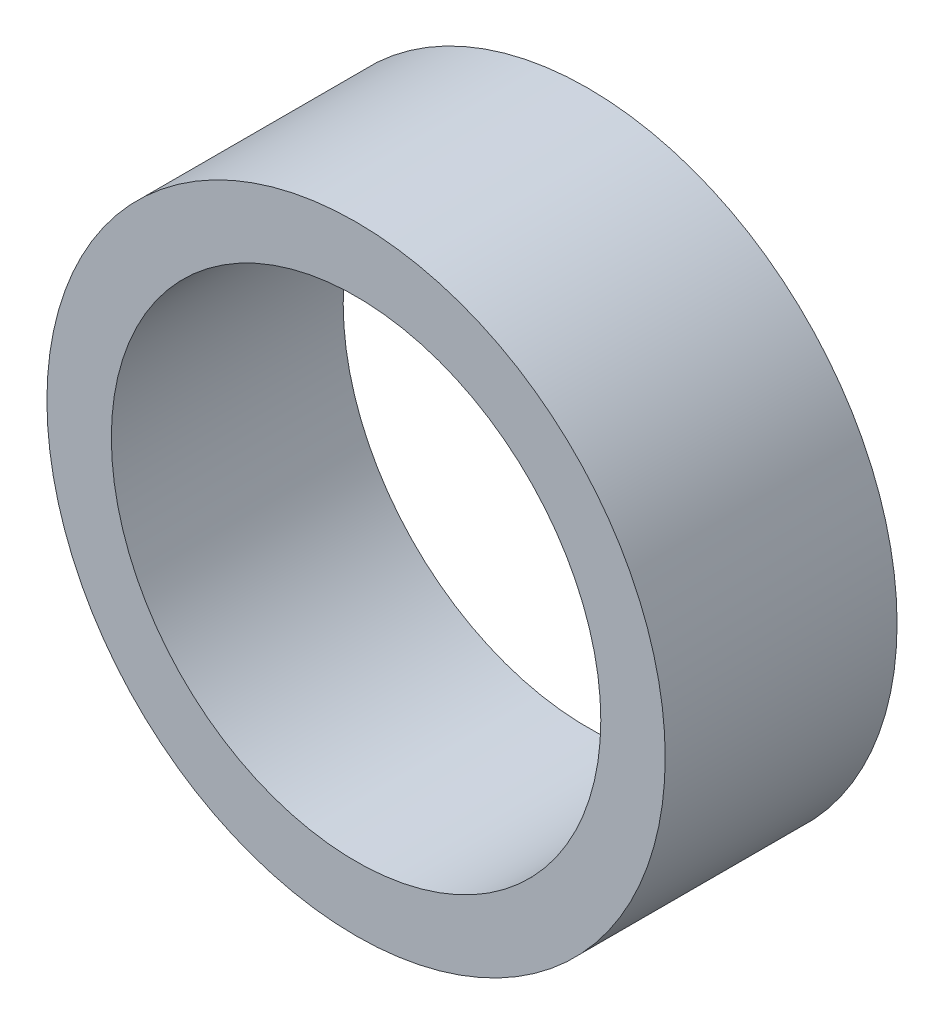
SolidWorks part; units mm, degrees
ref_plane "前视基准面" through (0, 0, 0) normal (0, 0, 1) x (1, 0, 0)
ref_plane "上视基准面" through (0, 0, 0) normal (0, 1, 0) x (1, 0, 0)
ref_plane "右视基准面" through (0, 0, 0) normal (1, 0, 0) x (0, 0, -1)
other "Configuration Table"
sketch "草图1" plane through (0, 0, 0) normal (0, 0, 1) x (1, 0, 0)
  circle A0 centre (0, 0) radius 19
  circle A1 centre (0, 0) radius 24
extrude "凸台-拉伸1" add sketch "草图1" along normal blind 18
